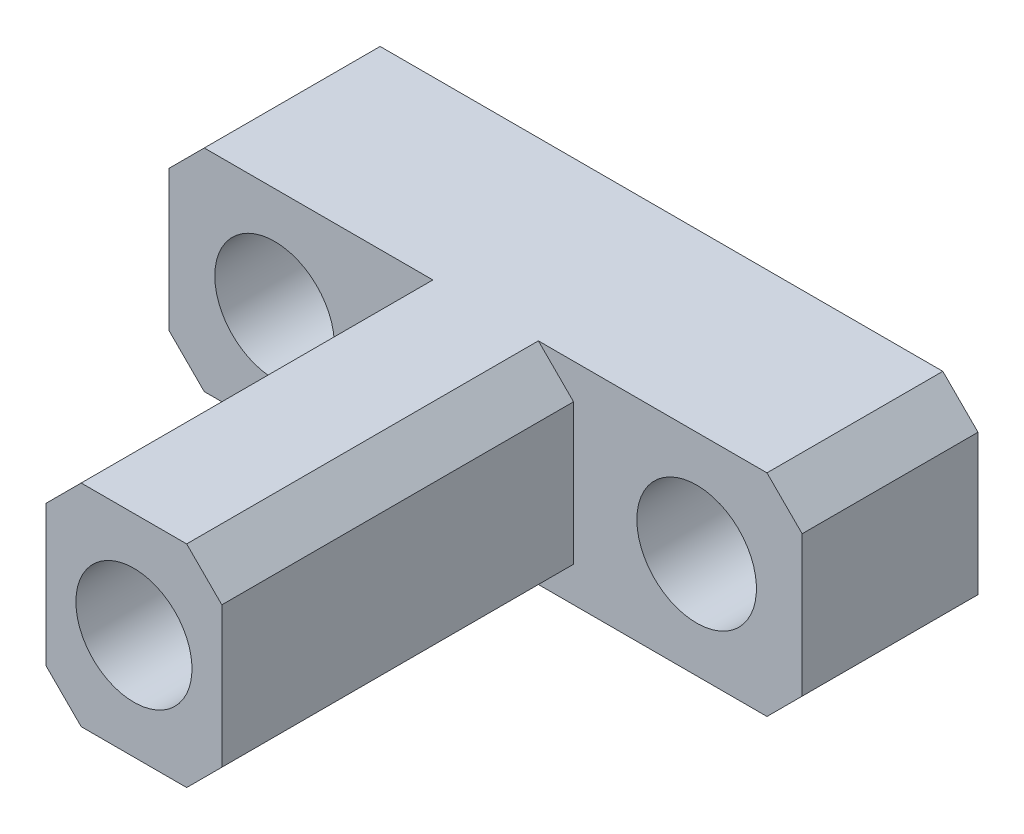
SolidWorks part; units mm, degrees
material "S45C"
ref_plane "Front Plane" through (0, 0, 0) normal (0, 0, 1) x (1, 0, 0)
ref_plane "Top Plane" through (0, 0, 0) normal (0, 1, 0) x (1, 0, 0)
ref_plane "Right Plane" through (0, 0, 0) normal (1, 0, 0) x (0, 0, -1)
sketch "Sketch3" plane through (0, 0, 0) normal (0, 1, 0) x (1, 0, 0)
  line L0 (0, 0) -> (0, -13.5704) construction
  line L1 (-9, -7.5) -> (9, -7.5)
  line L2 (-9, -7.5) -> (-9, 7.5)
  line L3 (-9, 7.5) -> (9, 7.5)
  line L4 (9, -7.5) -> (9, 7.5)
  line L5 (-9, -7.5) -> (9, 7.5) construction
  line L6 (-9, 7.5) -> (9, -7.5) construction
  point P0 (0, 0)
  dimension "D1" = 15
  dimension "D2" = 18
extrude "Boss-Extrude2" add sketch "Sketch3" along normal mid plane 6
hole_wizard "M3 Clearance Hole1" positions "Sketch5" profile "Sketch6" hole size "M3" standard "GB" end condition through all
sketch "Sketch5" plane through (0, 0, -7.5) normal (0, 0, -1) x (-1, 0, 0)
  line L0 (0, 0) -> (0, -7.986) construction
  point P0 (-6, 0)
  point P3 (6, 0)
  dimension "D1" = 12
sketch "Sketch6" plane through (6, 0, -7.5) normal (1, 0, 0) x (0, 1, 0)
  line L0 (0, 0) -> (0, 15)
  line L1 (0, 15) -> (1.7, 15)
  line L2 (1.7, 15) -> (1.7, 0)
  line L5 (1.7, 0) -> (0, 0)
  line L11 (0, -6.35) -> (0, 107.95) construction
  dimension "通孔孔直径" = 3.4
  dimension "通孔孔深度" = 15
chamfer "Chamfer1" distance 1 angle 45 4 edges at (-9, 3, 0) (-9, -3, 0) (9, 3, 0) (9, -3, 0)
sketch "Sketch10" plane through (0, -3, 0) normal (0, -1, 0) x (-1, 0, 0)
  line L0 (0, 0) -> (0, -9.1113) construction
  line L1 (-9, -7.5) -> (-2.5, -7.5)
  line L2 (-9, -7.5) -> (-9, 2.5)
  line L3 (-9, 2.5) -> (-2.5, 2.5)
  line L4 (-2.5, -7.5) -> (-2.5, 2.5)
  line L5 (9, -7.5) -> (2.5, -7.5)
  line L6 (9, -7.5) -> (9, 2.5)
  line L7 (9, 2.5) -> (2.5, 2.5)
  line L8 (2.5, -7.5) -> (2.5, 2.5)
  line L10 (8, 7.5) -> (-8, 7.5) construction
  dimension "D1" = 6.5
  dimension "D2" = 5
extrude "Cut-Extrude1" cut sketch "Sketch10" against normal through all
hole_wizard "M4 Tapped Hole1" positions "Sketch8" profile "Sketch7" tap size "M4" standard "GB" end condition through all
sketch "Sketch8" plane through (0, 0, -7.5) normal (0, 0, -1) x (-1, 0, 0)
  point P0 (0, 0)
sketch "Sketch7" plane through (0, 0, -7.5) normal (1, 0, 0) x (0, 1, 0)
  line L0 (0, 0) -> (0, 15)
  line L1 (0, 15) -> (1.65, 15)
  line L2 (1.65, 15) -> (1.65, 0)
  line L5 (1.65, 0) -> (0, 0)
  line L11 (0, -6.35) -> (0, 107.95) construction
  dimension "通孔螺纹孔钻头直径" = 3.3
  dimension "通孔螺纹孔钻头深度" = 15
cosmetic thread "Hole Thread1" parameters "D2"=4
chamfer "Chamfer2" distance 1 angle 45 4 edges at (-2.5, 3, 2.5) (-2.5, -3, 2.5) (2.5, 3, 2.5) (2.5, -3, 2.5)
